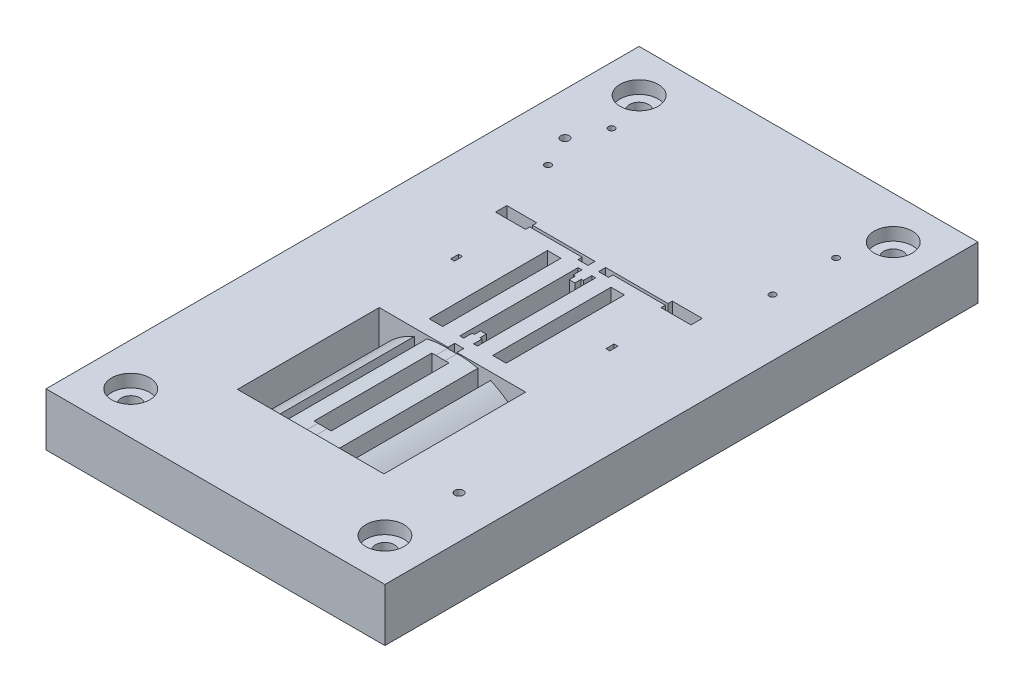
from build123d import *

# Parameters (mm, degrees)
SKETCH1_W                                        = 160
SKETCH1_H                                        = 280
BOSS_EXTRUDE1_DEPTH                              = 25
CBORE_FOR_M8_PAN_HEAD_MACHINE_SCREW1_D           = 9
CBORE_FOR_M8_PAN_HEAD_MACHINE_SCREW1_CBORE_D     = 18
CBORE_FOR_M8_PAN_HEAD_MACHINE_SCREW1_CBORE_DEPTH = 6
CUT_EXTRUDE2_DEPTH                               = 72.8
CUT_EXTRUDE4_REACH                               = 294.276
SKETCH_5_W                                       = 4.24
SKETCH_5_H                                       = 3.34
SKETCH_5_W_2                                     = 8.12
SKETCH_5_H_2                                     = 55.62
SKETCH_5_W_3                                     = 1.84
SKETCH_5_H_3                                     = 3.84
SKETCH_5_W_4                                     = 6.34
SKETCH_5_H_4                                     = 55.84
SKETCH_6_W                                       = 6
SKETCH_6_H                                       = 72.8
CUT_EXTRUDE5_DEPTH                               = 15
EXTRUDE_1_DEPTH                                  = 5.9
SKETCH10_R                                       = 2.5
CUT_EXTRUDE6_DEPTH                               = 20
SKETCH13_R                                       = 1.5
CUT_EXTRUDE7_DEPTH                               = 8
SKETCH14_R                                       = 2
CUT_EXTRUDE8_DEPTH                               = 293.275554914


with BuildPart() as part:
    # Sketch1 → Boss-Extrude1 (new body)
    with BuildSketch(Plane(origin=(0, 0, 0), x_dir=(1, 0, 0), z_dir=(0, 1, 0))):
        with Locations((0, -140)):
            Rectangle(SKETCH1_W, SKETCH1_H)
    extrude(amount=-BOSS_EXTRUDE1_DEPTH)

    # CBORE for M8 Pan Head Machine Screw1 (through all)
    with Locations(Plane(origin=(0, 0, 0), x_dir=(1, 0, 0), z_dir=(0, 1, 0))):
        with Locations((-60, -260), (60, -260), (60, -20), (-60, -20)):
            CounterBoreHole(CBORE_FOR_M8_PAN_HEAD_MACHINE_SCREW1_D / 2, CBORE_FOR_M8_PAN_HEAD_MACHINE_SCREW1_CBORE_D / 2, CBORE_FOR_M8_PAN_HEAD_MACHINE_SCREW1_CBORE_DEPTH)

    # Sketch4 → Cut-Extrude2 (cut)
    with BuildSketch(Plane.XY.offset(240.93)):
        with BuildLine():
            ThreePointArc((29.525310886, -11.154947057), (16.931588105, -3.095666176), (2.206902067, -0.5))
            Line((2.206902067, -0.5), (-2.206902067, -0.5))
            ThreePointArc((-2.206902067, -0.5), (-16.931588105, -3.095666176), (-29.525310886, -11.154947057))
            Line((-29.525310886, -11.154947057), (-29.525310886, -19.27))
            ThreePointArc((-29.525310886, -19.27), (-29.890310886, -19.902198545), (-30.620310886, -19.902198545))
            Line((-30.620310886, -19.902198545), (-34.572188183, -17.620581124))
            Line((-34.572188183, -17.620581124), (-34.572188183, 0))
            Line((-34.572188183, 0), (34.572188183, 0))
            Line((34.572188183, 0), (34.572188183, -17.620581124))
            Line((34.572188183, -17.620581124), (30.620310886, -19.902198545))
            ThreePointArc((30.620310886, -19.902198545), (29.890310886, -19.902198545), (29.525310886, -19.27))
            Line((29.525310886, -19.27), (29.525310886, -11.154947057))
        make_face()
    extrude(amount=-CUT_EXTRUDE2_DEPTH, mode=Mode.SUBTRACT)

    # 草图5 → Cut-Extrude4 (cut, up to next)
    with BuildSketch(Plane(origin=(0, 0, 0), x_dir=(1, 0, 0), z_dir=(0, 1, 0)), mode=Mode.PRIVATE) as cut_extrude4_sk1:
        with Locations((0, -166.58)):
            Rectangle(SKETCH_5_W, SKETCH_5_H)
    cut_extrude4_tool1 = extrude(cut_extrude4_sk1.sketch, amount=-CUT_EXTRUDE4_REACH, mode=Mode.PRIVATE) & part.part
    # 草图5 → Cut-Extrude4 (cut, up to next)
    with BuildSketch(Plane(origin=(0, 0, 0), x_dir=(1, 0, 0), z_dir=(0, 1, 0)), mode=Mode.PRIVATE) as cut_extrude4_sk2:
        with Locations((0, -201.61)):
            Rectangle(SKETCH_5_W_2, SKETCH_5_H_2)
    cut_extrude4_tool2 = extrude(cut_extrude4_sk2.sketch, amount=-CUT_EXTRUDE4_REACH, mode=Mode.PRIVATE) & part.part
    # 草图5 → Cut-Extrude4 (cut, up to next)
    with BuildSketch(Plane(origin=(0, 0, 0), x_dir=(1, 0, 0), z_dir=(0, 1, 0)), mode=Mode.PRIVATE) as cut_extrude4_sk3:
        with Locations((36.69, -129.5)):
            Rectangle(SKETCH_5_W_3, SKETCH_5_H_3)
    cut_extrude4_tool3 = extrude(cut_extrude4_sk3.sketch, amount=-CUT_EXTRUDE4_REACH, mode=Mode.PRIVATE) & part.part
    # 草图5 → Cut-Extrude4 (cut, up to next)
    with BuildSketch(Plane(origin=(0, 0, 0), x_dir=(1, 0, 0), z_dir=(0, 1, 0)), mode=Mode.PRIVATE) as cut_extrude4_sk4:
        with Locations((15, -133)):
            Rectangle(SKETCH_5_W_4, SKETCH_5_H_4)
    cut_extrude4_tool4 = extrude(cut_extrude4_sk4.sketch, amount=-CUT_EXTRUDE4_REACH, mode=Mode.PRIVATE) & part.part
    # 草图5 → Cut-Extrude4 (cut, up to next)
    with BuildSketch(Plane(origin=(0, 0, 0), x_dir=(1, 0, 0), z_dir=(0, 1, 0)), mode=Mode.PRIVATE) as cut_extrude4_sk5:
        Polygon((4.39, -104.86), (4.39, -160.7), (2.55, -160.7), (2.55, -156.7), (1.55, -156.7), (1.55, -153.7), (-1.11, -153.7), (-1.11, -156.7), (-2.11, -156.7), (-2.11, -160.7), (-3.95, -160.7), (-3.95, -104.86), (-2.11, -104.86), (-2.11, -108.86), (-1.11, -108.86), (-1.11, -111.86), (1.55, -111.86), (1.55, -108.86), (2.55, -108.86), (2.55, -104.86), align=None)
    cut_extrude4_tool5 = extrude(cut_extrude4_sk5.sketch, amount=-CUT_EXTRUDE4_REACH, mode=Mode.PRIVATE) & part.part
    # 草图5 → Cut-Extrude4 (cut, up to next)
    with BuildSketch(Plane(origin=(0, 0, 0), x_dir=(1, 0, 0), z_dir=(0, 1, 0)), mode=Mode.PRIVATE) as cut_extrude4_sk6:
        with Locations((-15, -133)):
            Rectangle(SKETCH_5_W_4, SKETCH_5_H_4)
    cut_extrude4_tool6 = extrude(cut_extrude4_sk6.sketch, amount=-CUT_EXTRUDE4_REACH, mode=Mode.PRIVATE) & part.part
    # 草图5 → Cut-Extrude4 (cut, up to next)
    with BuildSketch(Plane(origin=(0, 0, 0), x_dir=(1, 0, 0), z_dir=(0, 1, 0)), mode=Mode.PRIVATE) as cut_extrude4_sk7:
        with Locations((-36.69, -129.5)):
            Rectangle(SKETCH_5_W_3, SKETCH_5_H_3)
    cut_extrude4_tool7 = extrude(cut_extrude4_sk7.sketch, amount=-CUT_EXTRUDE4_REACH, mode=Mode.PRIVATE) & part.part
    # 草图5 → Cut-Extrude4 (cut, up to next)
    with BuildSketch(Plane(origin=(0, 0, 0), x_dir=(1, 0, 0), z_dir=(0, 1, 0)), mode=Mode.PRIVATE) as cut_extrude4_sk8:
        Polygon((7.25, -101.64), (2.5, -101.64), (2.5, -98.3), (31.99, -98.3), (31.99, -96.3), (46.14, -96.3), (46.14, -101.64), (31.99, -101.64), (31.99, -99.64), (7.25, -99.64), align=None)
    cut_extrude4_tool8 = extrude(cut_extrude4_sk8.sketch, amount=-CUT_EXTRUDE4_REACH, mode=Mode.PRIVATE) & part.part
    # 草图5 → Cut-Extrude4 (cut, up to next)
    with BuildSketch(Plane(origin=(0, 0, 0), x_dir=(1, 0, 0), z_dir=(0, 1, 0)), mode=Mode.PRIVATE) as cut_extrude4_sk9:
        Polygon((-2.5, -98.3), (-31.99, -98.3), (-31.99, -96.3), (-46.14, -96.3), (-46.14, -101.64), (-31.99, -101.64), (-31.99, -99.64), (-7.25, -99.64), (-7.25, -101.64), (-2.5, -101.64), align=None)
    cut_extrude4_tool9 = extrude(cut_extrude4_sk9.sketch, amount=-CUT_EXTRUDE4_REACH, mode=Mode.PRIVATE) & part.part
    add(cut_extrude4_tool1.solids().sort_by_distance((0, 0, 166.58))[0], mode=Mode.SUBTRACT)
    add(cut_extrude4_tool2.solids().sort_by_distance((0, 0, 201.61))[0], mode=Mode.SUBTRACT)
    add(cut_extrude4_tool3.solids().sort_by_distance((36.69, 0, 129.5))[0], mode=Mode.SUBTRACT)
    add(cut_extrude4_tool4.solids().sort_by_distance((15, 0, 133))[0], mode=Mode.SUBTRACT)
    add(cut_extrude4_tool5.solids().sort_by_distance((0.22, 0, 132.78))[0], mode=Mode.SUBTRACT)
    add(cut_extrude4_tool6.solids().sort_by_distance((-15, 0, 133))[0], mode=Mode.SUBTRACT)
    add(cut_extrude4_tool7.solids().sort_by_distance((-36.69, 0, 129.5))[0], mode=Mode.SUBTRACT)
    add(cut_extrude4_tool8.solids().sort_by_distance((29.536343, 0, 99.09735))[0], mode=Mode.SUBTRACT)
    add(cut_extrude4_tool9.solids().sort_by_distance((-29.536343, 0, 99.09735))[0], mode=Mode.SUBTRACT)

    # 草图6 → Cut-Extrude5 (cut)
    with BuildSketch(Plane(origin=(0, 0, 0), x_dir=(1, 0, 0), z_dir=(0, 1, 0))):
        with Locations((-15, -204.53)):
            Rectangle(SKETCH_6_W, SKETCH_6_H)
        with Locations((15, -204.53)):
            Rectangle(SKETCH_6_W, SKETCH_6_H)
    extrude(amount=-CUT_EXTRUDE5_DEPTH, mode=Mode.SUBTRACT)

    # Sketch7 → 凸台-拉伸1 (add)
    with BuildSketch(Plane(origin=(0, 0, 240.93), x_dir=(-1, 0, 0), z_dir=(0, 0, -1))):
        with BuildLine():
            Line((-18, -3.531117464), (-18, -15))
            Line((-18, -15), (-12, -15))
            Line((-12, -15), (-12, -1.548321679))
            ThreePointArc((-12, -1.548321679), (-7.137450284, -0.706550326), (-2.206902067, -0.5))
            Line((-2.206902067, -0.5), (2.206902067, -0.5))
            ThreePointArc((2.206902067, -0.5), (7.137450284, -0.706550326), (12, -1.548321679))
            Line((12, -1.548321679), (12, -15))
            Line((12, -15), (18, -15))
            Line((18, -15), (18, -3.531117464))
            ThreePointArc((18, -3.531117464), (24.110999277, -6.816424086), (29.525310886, -11.154947057))
            Line((29.525310886, -11.154947057), (29.525310886, -19.27))
            ThreePointArc((29.525310886, -19.27), (29.890310886, -19.902198545), (30.620310886, -19.902198545))
            Line((30.620310886, -19.902198545), (34.572188183, -17.620581124))
            Line((34.572188183, -17.620581124), (34.572188183, 0))
            Line((34.572188183, 0), (-34.572188183, 0))
            Line((-34.572188183, 0), (-34.572188183, -17.620581124))
            Line((-34.572188183, -17.620581124), (-30.620310886, -19.902198545))
            ThreePointArc((-30.620310886, -19.902198545), (-29.890310886, -19.902198545), (-29.525310886, -19.27))
            Line((-29.525310886, -19.27), (-29.525310886, -11.154947057))
            ThreePointArc((-29.525310886, -11.154947057), (-24.110999277, -6.816424086), (-18, -3.531117464))
        make_face()
    extrude(amount=EXTRUDE_1_DEPTH)

    # Sketch10 → Cut-Extrude6 (cut)
    with BuildSketch(Plane(origin=(0, 0, 0), x_dir=(1, 0, 0), z_dir=(0, 1, 0))):
        with Locations(Location((-15, -184.86, 0), (0, 0, 270))):
            Circle(SKETCH10_R)
        with Locations(Location((-15, -218.315, 0), (0, 0, 270))):
            Circle(SKETCH10_R)
        with Locations(Location((-15, -201.585, 0), (0, 0, 270))):
            Circle(SKETCH10_R)
        with Locations(Location((15, -218.315, 0), (0, 0, 90))):
            Circle(SKETCH10_R)
        with Locations(Location((15, -201.585, 0), (0, 0, 90))):
            Circle(SKETCH10_R)
        with Locations(Location((15, -184.86, 0), (0, 0, 90))):
            Circle(SKETCH10_R)
    extrude(amount=-CUT_EXTRUDE6_DEPTH, mode=Mode.SUBTRACT)

    # Sketch13 → Cut-Extrude7 (cut)
    with BuildSketch(Plane(origin=(0, 0, 0), x_dir=(1, 0, 0), z_dir=(0, 1, 0))):
        with Locations(Location((-53.003, -40, 0), (0, 0, 270))):
            Circle(SKETCH13_R)
        with Locations(Location((-53.003, -69.996579655, 0), (0, 0, 270))):
            Circle(SKETCH13_R)
        with Locations(Location((53.003, -69.996579655, 0), (0, 0, 90))):
            Circle(SKETCH13_R)
        with Locations(Location((53.003, -40, 0), (0, 0, 90))):
            Circle(SKETCH13_R)
        Polygon((7.25, -99.64), (31.99, -99.64), (31.99, -101.64), (46.14, -101.64), (46.14, -96.3), (31.99, -96.3), (31.99, -98.3), (2.5, -98.3), (2.5, -101.64), (7.25, -101.64), align=None)
        Polygon((-2.5, -98.3), (-31.99, -98.3), (-31.99, -96.3), (-46.14, -96.3), (-46.14, -101.64), (-31.99, -101.64), (-31.99, -99.64), (-7.25, -99.64), (-7.25, -101.64), (-2.5, -101.64), align=None)
    extrude(amount=-CUT_EXTRUDE7_DEPTH, mode=Mode.SUBTRACT)

    # Sketch14 → Cut-Extrude8 (cut, through all)
    with BuildSketch(Plane.XZ.offset(25)):
        with Locations(Location((-60, 55, 0), (0, 0, 270))):
            Circle(SKETCH14_R)
        with Locations(Location((60, 225, 0), (0, 0, 270))):
            Circle(SKETCH14_R)
    extrude(amount=-CUT_EXTRUDE8_DEPTH, mode=Mode.SUBTRACT)


solid = part.part
